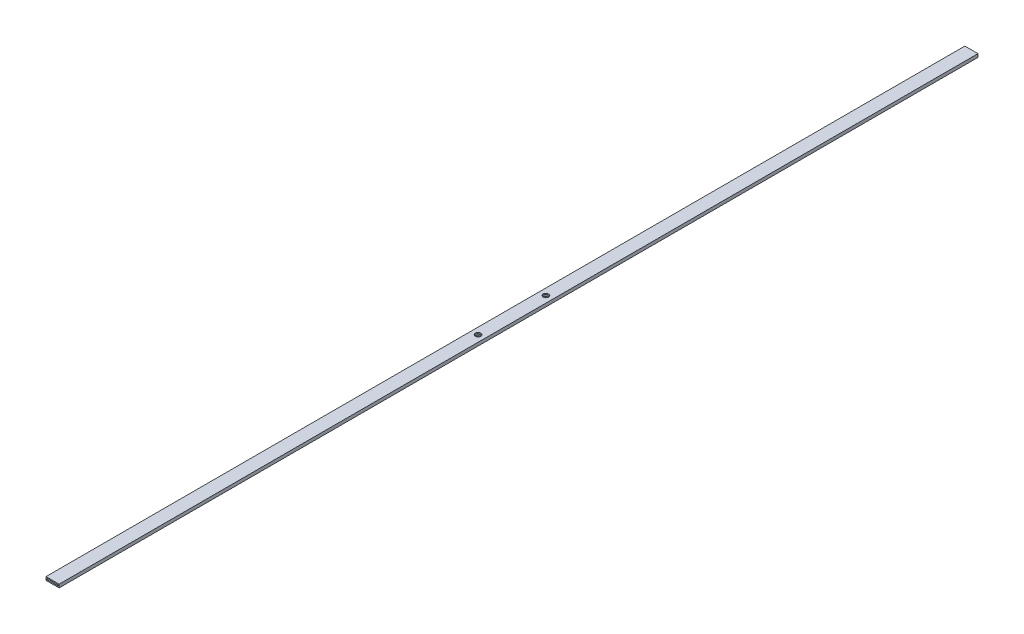
from build123d import *

# Parameters (mm, degrees)
SKETCH1_W             = 12
SKETCH1_H             = 3
BOSS_EXTRUDE1_DEPTH   = 840
SKETCH2_W             = 10
SKETCH2_H             = 1
CUT_EXTRUDE1_DEPTH    = 841.951655259
M6_TAPPED_HOLE1_D     = 5
M6_TAPPED_HOLE1_DEPTH = 15
M6_TAPPED_HOLE1_TIP   = 1.502151548


with BuildPart() as part:
    # Sketch1 → Boss-Extrude1 (new body)
    with BuildSketch(Plane.XY):
        with Locations((-25.901003365, 22.624934563)):
            Rectangle(SKETCH1_W, SKETCH1_H)
    extrude(amount=BOSS_EXTRUDE1_DEPTH)

    # Sketch2 → Cut-Extrude1 (cut, through all)
    with BuildSketch(Plane.XY.offset(840)):
        with Locations((-25.901003365, 22.624934563)):
            Rectangle(SKETCH2_W, SKETCH2_H)
    extrude(amount=-CUT_EXTRUDE1_DEPTH, mode=Mode.SUBTRACT)

    # M6 Tapped Hole1
    with Locations(Plane(origin=(-25.901003365, 24.124934563, 389), x_dir=(0, 0, 1), z_dir=(0, 1, 0))):
        with Locations((0, 0), (62, 0)):
            Hole(M6_TAPPED_HOLE1_D / 2, depth=M6_TAPPED_HOLE1_DEPTH)
            with Locations((0, 0, -(M6_TAPPED_HOLE1_DEPTH + M6_TAPPED_HOLE1_TIP / 2))):  # 118° drill point
                Cone(0, M6_TAPPED_HOLE1_D / 2, M6_TAPPED_HOLE1_TIP, mode=Mode.SUBTRACT)


solid = part.part
